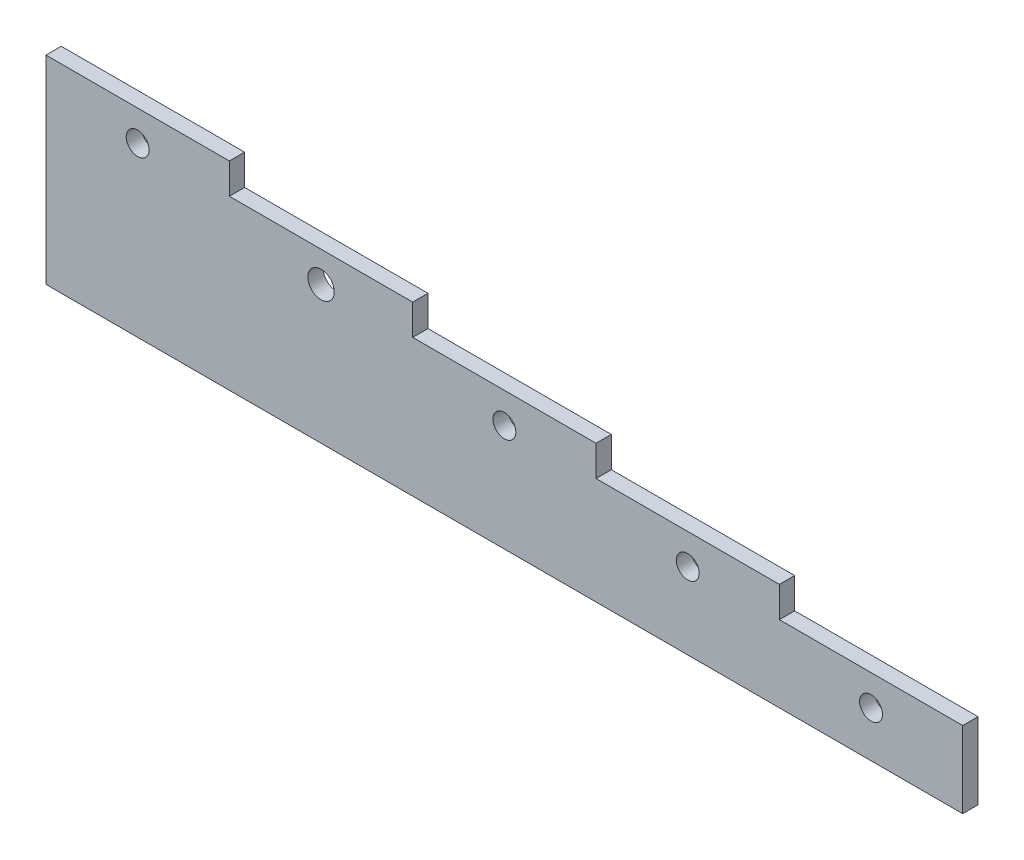
SolidWorks part; units mm, degrees
ref_plane "Front Plane" through (0, 0, 0) normal (0, 0, 1) x (1, 0, 0)
ref_plane "Top Plane" through (0, 0, 0) normal (0, 1, 0) x (1, 0, 0)
ref_plane "Right Plane" through (0, 0, 0) normal (1, 0, 0) x (0, 0, -1)
sketch "Sketch1" plane through (0, 0, 0) normal (0, 0, 1) x (1, 0, 0)
  line L0 (0, 0) -> (600, 0)
  line L1 (600, 0) -> (600, 50)
  line L2 (600, 50) -> (480, 50)
  line L3 (480, 50) -> (480, 70)
  line L4 (480, 70) -> (360, 70)
  line L5 (360, 70) -> (360, 90)
  line L6 (360, 90) -> (240, 90)
  line L7 (240, 90) -> (240, 110)
  line L8 (240, 110) -> (120, 110)
  line L9 (120, 110) -> (120, 130)
  line L10 (120, 130) -> (0, 130)
  line L11 (0, 130) -> (0, 0)
  circle A0 centre (60, 110) radius 7.5
  circle A1 centre (180, 90) radius 8.6524
  circle A2 centre (300, 70) radius 7.5
  circle A3 centre (420, 50) radius 7.5
  circle A4 centre (540, 30) radius 7.5
  dimension "D13" = 15
  dimension "D14" = 20
  dimension "D15" = 60
  dimension "D16" = 20
  dimension "D17" = 15
  dimension "D18" = 15
  dimension "D19" = 15
  dimension "D1" = 600
  dimension "D2" = 120
  dimension "D3" = 120
  dimension "D4" = 120
  dimension "D6" = 50
  dimension "D7" = 20
  dimension "D10" = 20
  dimension "D11" = 120
  dimension "D12" = 20
extrude "Boss-Extrude1" add sketch "Sketch1" along normal blind 10
